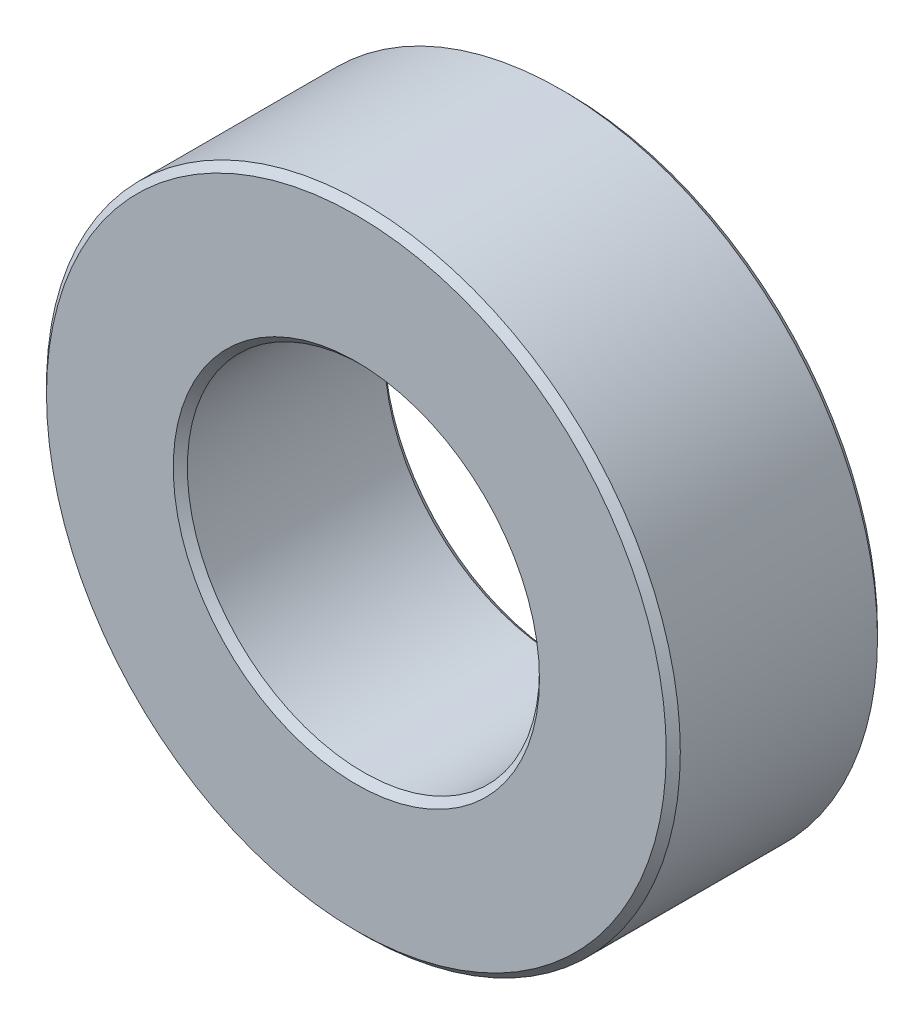
from build123d import *

# Parameters (mm, degrees)
SKETCH1_R           = 90
SKETCH1_R_2         = 50
BOSS_EXTRUDE1_DEPTH = 60
CHAMFER1_SIZE       = 2


with BuildPart() as part:
    # Sketch1 → Boss-Extrude1 (new body)
    with BuildSketch(Plane.XY):
        Circle(SKETCH1_R)
        Circle(SKETCH1_R_2, mode=Mode.SUBTRACT)
    extrude(amount=BOSS_EXTRUDE1_DEPTH)

    # Chamfer1
    chamfer1_edges = [part.edges().sort_by_distance(p)[0] for p in [
        (-90, 0, 0),
        (-90, 0, 60),
        (-50, 0, 0),
        (-50, 0, 60),
    ]]
    chamfer(chamfer1_edges, length=CHAMFER1_SIZE)


solid = part.part
